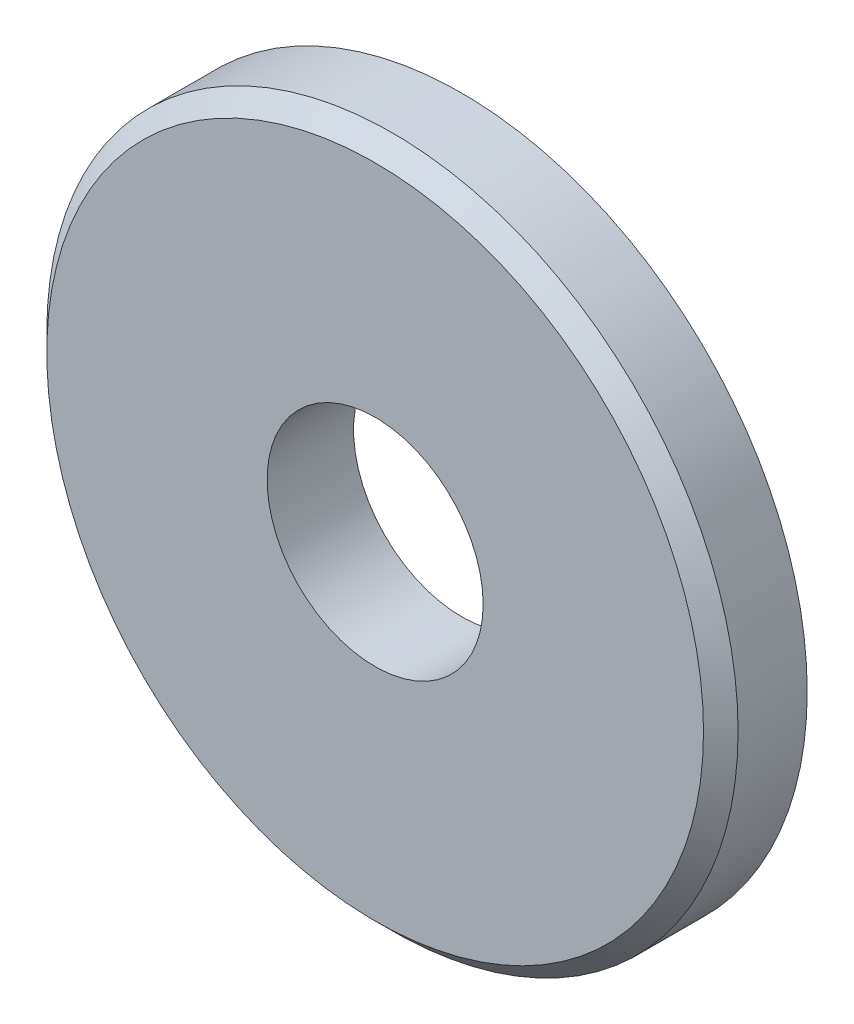
from build123d import *

# Parameters (mm, degrees)
SKETCH_1_R      = 20
SKETCH_1_R_2    = 6.25
EXTRUDE_1_DEPTH = 5
CHAMFER_1_SIZE  = 1


with BuildPart() as part:
    # 草图1 → 凸台-拉伸1 (new body)
    with BuildSketch(Plane.XY):
        Circle(SKETCH_1_R)
        Circle(SKETCH_1_R_2, mode=Mode.SUBTRACT)
    extrude(amount=EXTRUDE_1_DEPTH)

    # 倒角1
    chamfer_1_edges = [part.edges().sort_by_distance(p)[0] for p in [
        (-20, 0, 5),
    ]]
    chamfer(chamfer_1_edges, length=CHAMFER_1_SIZE)


solid = part.part
